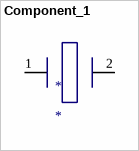
[diagram p0: symbol Component_1]
# Altium schematic symbol library MISC89340-23.SchLib: 1 symbol
Pins are listed as number, name and electrical type; pins without a type are passive.


## Component_1
designator *
footprint LC-HC-49S
pins: 1, 2